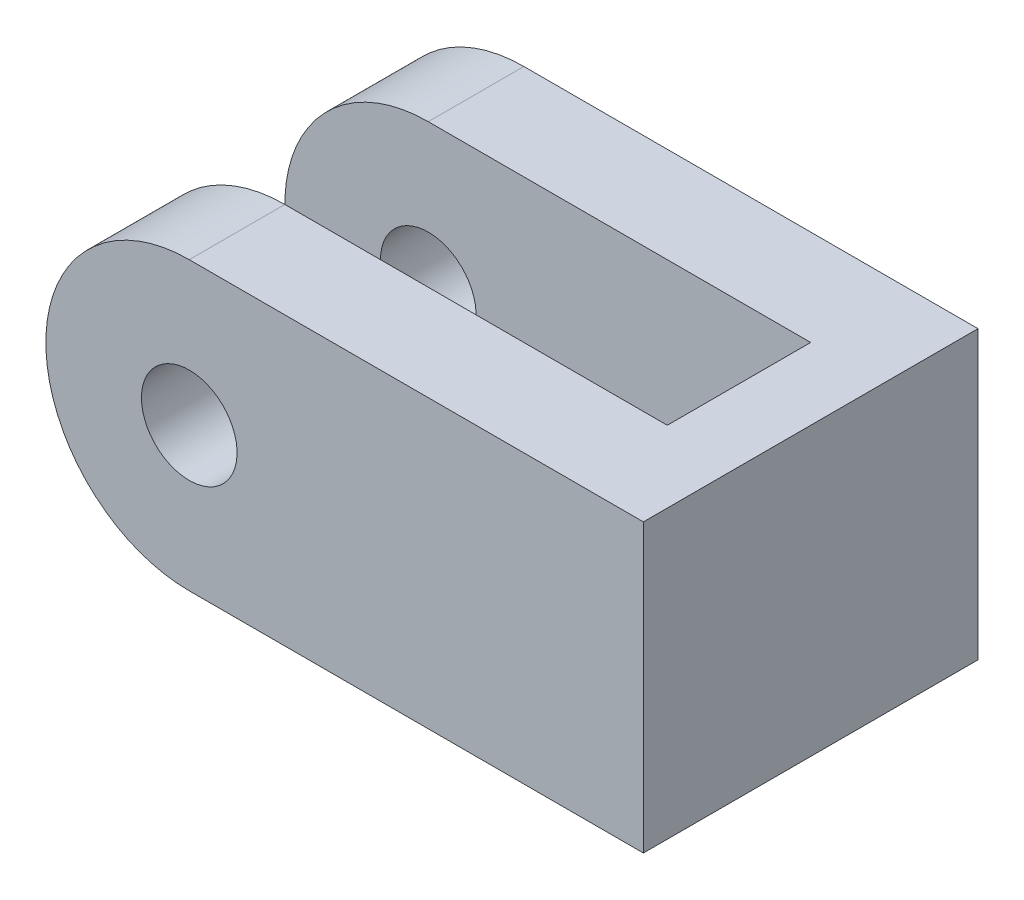
from build123d import *

# Parameters (mm, degrees)
BOSS_EXTRUDE1_DEPTH = 20
SKETCH2_R           = 10
CUT_EXTRUDE1_DEPTH  = 79.74007874
SKETCH3_W           = 35
SKETCH3_H           = 60
BOSS_EXTRUDE5_DEPTH = 15


with BuildPart() as part:
    # Sketch1 → Boss-Extrude1 (new body)
    with BuildSketch(Plane.XY):
        with BuildLine():
            Line((-40, 30), (40, 30))
            Line((40, 30), (40, -30))
            Line((40, -30), (-40, -30))
            ThreePointArc((-40, -30), (-70, 0), (-40, 30))
        make_face()
    extrude(amount=BOSS_EXTRUDE1_DEPTH)

    # Sketch2 → Cut-Extrude1 (cut, through all)
    with BuildSketch(Plane(origin=(0, 0, 0), x_dir=(-1, 0, 0), z_dir=(0, 0, -1))):
        with Locations((40, 0)):
            Circle(SKETCH2_R)
    extrude(amount=-CUT_EXTRUDE1_DEPTH, mode=Mode.SUBTRACT)

    # Sketch3 → Boss-Extrude5 (add)
    with BuildSketch(Plane(origin=(40, 0, 0), x_dir=(0, 0, -1), z_dir=(1, 0, 0))):
        with Locations((-2.5, 0)):
            Rectangle(SKETCH3_W, SKETCH3_H)
    extrude(amount=BOSS_EXTRUDE5_DEPTH)

    # Mirror1: part across plane


with BuildPart() as part_1:
    add(part.part)
    add(part.part.mirror(Plane(origin=(55, -30, -15), x_dir=(1, 0, 0), z_dir=(0, 0, 1))))


solid = part_1.part
